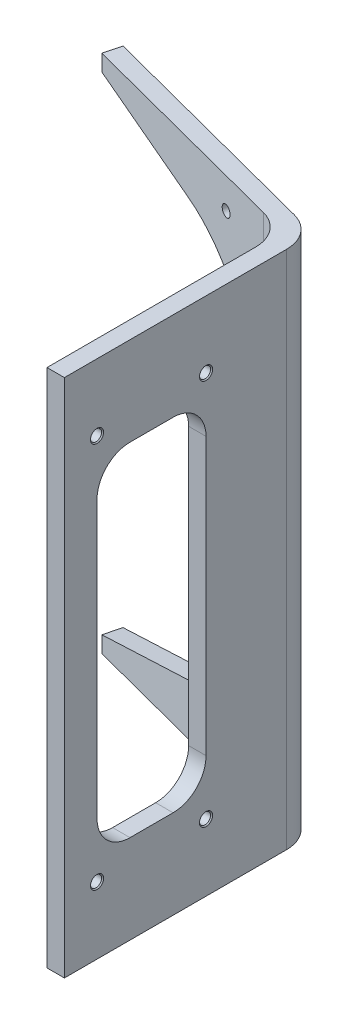
from build123d import *

# Parameters (mm, degrees)
BOSS_EXTRUDE1_DEPTH          = 478
CUT_EXTRUDE1_DEPTH           = 478
M12_TAPPED_HOLE1_D           = 10.2
M12_TAPPED_HOLE1_CSINK_D     = 12.05
M12_TAPPED_HOLE1_CSINK_ANGLE = 90
CUT_EXTRUDE2_DEPTH           = 478
M12_TAPPED_HOLE2_D           = 10.2
M12_TAPPED_HOLE2_CSINK_D     = 12.05
M12_TAPPED_HOLE2_CSINK_ANGLE = 90


with BuildPart() as part:
    # Sketch1 → Boss-Extrude1 (new body)
    with BuildSketch(Plane(origin=(0, 0, 0), x_dir=(1, 0, 0), z_dir=(0, 1, 0))):
        with BuildLine():
            Line((2489.747313266, 1503.388237), (2505.747313266, 1503.388237))
            Line((2505.747313266, 1503.388237), (2505.747313266, 1707.687544505))
            ThreePointArc((2505.747313266, 1707.687544505), (2499.07328063, 1727.247589931), (2481.835102198, 1738.648611511))
            Line((2481.835102198, 1738.648611511), (2268.738706702, 1794.314608702))
            Line((2268.738706702, 1794.314608702), (2264.694812236, 1778.834075199))
            Line((2264.694812236, 1778.834075199), (2465.835102198, 1726.291305576))
            ThreePointArc((2465.835102198, 1726.291305576), (2483.07328063, 1714.890283996), (2489.747313266, 1695.33023857))
            Line((2489.747313266, 1695.33023857), (2489.747313266, 1503.388237))
        make_face()
    extrude(amount=BOSS_EXTRUDE1_DEPTH)

    # Sketch2 → Cut-Extrude1 (cut)
    with BuildSketch(Plane(origin=(2505.747313266, 0, 0), x_dir=(0, 0, -1), z_dir=(1, 0, 0))):
        with BuildLine():
            Line((1563.688237, 81.6), (1603.288237, 81.6))
            ThreePointArc((1603.288237, 81.6), (1624.71357247, 90.47466453), (1633.588237, 111.9))
            Line((1633.588237, 111.9), (1633.588237, 366.1))
            ThreePointArc((1633.588237, 366.1), (1624.71357247, 387.52533547), (1603.288237, 396.4))
            Line((1603.288237, 396.4), (1563.688237, 396.4))
            ThreePointArc((1563.688237, 396.4), (1542.26290153, 387.52533547), (1533.388237, 366.1))
            Line((1533.388237, 366.1), (1533.388237, 111.9))
            ThreePointArc((1533.388237, 111.9), (1542.26290153, 90.47466453), (1563.688237, 81.6))
        make_face()
    extrude(amount=-CUT_EXTRUDE1_DEPTH, mode=Mode.SUBTRACT)

    # M12 Tapped Hole1 (through all)
    with Locations(Plane(origin=(2505.747313266, 0, 0), x_dir=(0, 0, -1), z_dir=(1, 0, 0))):
        with Locations((1633.588237, 416.55), (1533.388237, 61.45), (1533.388237, 416.55), (1633.588237, 61.45)):
            CounterSinkHole(M12_TAPPED_HOLE1_D / 2, M12_TAPPED_HOLE1_CSINK_D / 2, counter_sink_angle=M12_TAPPED_HOLE1_CSINK_ANGLE)

    # Sketch7 → Cut-Extrude2 (cut)
    with BuildSketch(Plane(origin=(583.702793267, 0, -2234.487255477), x_dir=(-0.9675333439556839, 0, -0.2527434041353648), z_dir=(0.2527434041353648, 0, -0.967533343955684))):
        with BuildLine():
            Line((-1741.579165164, 463), (-1741.579165164, 15))
            Line((-1741.579165164, 15), (-1853.078764419, 46.9719956))
            ThreePointArc((-1853.078764419, 46.9719956), (-1910.190162861, 86.223572269), (-1932.179165164, 151.941772797))
            Line((-1932.179165164, 151.941772797), (-1932.179165164, 326.058227203))
            ThreePointArc((-1932.179165164, 326.058227203), (-1910.190162861, 391.776427731), (-1853.078764419, 431.0280044))
            Line((-1853.078764419, 431.0280044), (-1741.579165164, 463))
        make_face()
    extrude(amount=-CUT_EXTRUDE2_DEPTH, mode=Mode.SUBTRACT)

    # M12 Tapped Hole2 (through all)
    with Locations(Plane(origin=(583.702793267, 0, -2234.487255477), x_dir=(-0.9675333439556839, 0, -0.2527434041353648), z_dir=(0.2527434041353648, 0, -0.967533343955684))):
        with Locations((-1901.479165164, 450), (-1901.479165164, 28)):
            CounterSinkHole(M12_TAPPED_HOLE2_D / 2, M12_TAPPED_HOLE2_CSINK_D / 2, counter_sink_angle=M12_TAPPED_HOLE2_CSINK_ANGLE)


solid = part.part
